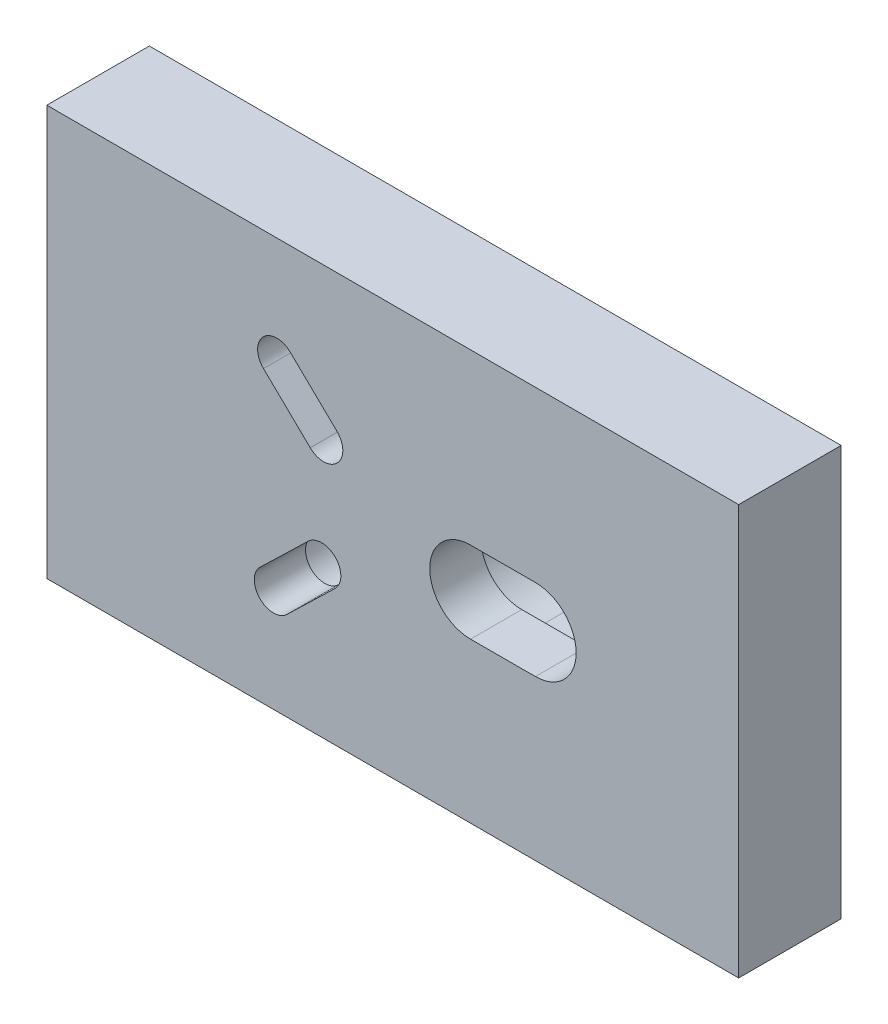
from build123d import *

# Parameters (mm, degrees)
SKETCH_1_W          = 27
SKETCH_1_H          = 16
EXTRUDE_1_DEPTH     = 4
SKETCH_2_R          = 0.75
SKETCH_2_R_2        = 1.59
CUT_EXTRUDE_2_DEPTH = 4
CUT_EXTRUDE_3_DEPTH = 4
CUT_EXTRUDE_4_DEPTH = 2


with BuildPart() as part:
    # 草图1 → 凸台-拉伸1 (new body)
    with BuildSketch(Plane.XY):
        with Locations((3.898916968, -3.881768953)):
            Rectangle(SKETCH_1_W, SKETCH_1_H)
    extrude(amount=EXTRUDE_1_DEPTH)

    # 草图2 → 切除-拉伸2 (cut)
    with BuildSketch(Plane.XY.offset(4)):
        with Locations((1.199905932, -1.781578746)):
            Circle(SKETCH_2_R)
        with Locations((1.122511443, -6.056778774)):
            Circle(SKETCH_2_R)
        with Locations((9.465404763, -4.069510677)):
            Circle(SKETCH_2_R_2)
    extrude(amount=-CUT_EXTRUDE_2_DEPTH, mode=Mode.SUBTRACT)

    # 草图3 → 切除-拉伸3 (cut)
    with BuildSketch(Plane.XY.offset(4)):
        with BuildLine():
            Line((6.931862452, -2.481455291), (9.464184068, -2.479511145))
            ThreePointArc((9.464184068, -2.479511145), (7.875405231, -4.070731371), (9.466625457, -5.659510208))
            Line((9.466625457, -5.659510208), (6.934303841, -5.661454354))
            ThreePointArc((6.934303841, -5.661454354), (5.343083615, -4.072675517), (6.931862452, -2.481455291))
        make_face()
        with BuildLine():
            Line((-1.276445305, -7.332757851), (0.601227077, -5.517554692))
            ThreePointArc((0.601227077, -5.517554692), (0.583287361, -6.578063139), (1.643795809, -6.596002856))
            Line((1.643795809, -6.596002856), (-0.233876574, -8.411206015))
            ThreePointArc((-0.233876574, -8.411206015), (-1.294385021, -8.393266299), (-1.276445305, -7.332757851))
        make_face()
        with BuildLine():
            Line((-1.145979965, -0.556904877), (0.678621567, -2.320802827))
            ThreePointArc((0.678621567, -2.320802827), (0.660681851, -1.26029438), (1.721190298, -1.242354664))
            Line((1.721190298, -1.242354664), (-0.103411234, 0.521543286))
            ThreePointArc((-0.103411234, 0.521543286), (-1.163919681, 0.50360357), (-1.145979965, -0.556904877))
        make_face()
    extrude(amount=-CUT_EXTRUDE_3_DEPTH, mode=Mode.SUBTRACT)

    # 草图5 → 切除-拉伸4 (cut)
    with BuildSketch(Plane(origin=(0, 0, 0), x_dir=(-1, 0, 0), z_dir=(0, 0, -1))):
        with BuildLine():
            Line((-9.463485432, -1.569511413), (-6.931163815, -1.57145556))
            ThreePointArc((-6.931163815, -1.57145556), (-4.433083883, -4.073374154), (-6.935002478, -6.571454086))
            Line((-6.935002478, -6.571454086), (-9.467324094, -6.56950994))
            ThreePointArc((-9.467324094, -6.56950994), (-11.965404026, -4.067591345), (-9.463485432, -1.569511413))
        make_face()
        with BuildLine():
            Line((-0.244111676, 0.881026007), (-2.068713208, -0.882871943))
            ThreePointArc((-2.068713208, -0.882871943), (-2.098612735, -2.650386022), (-0.331098657, -2.680285548))
            Line((-0.331098657, -2.680285548), (1.493502876, -0.916387599))
            ThreePointArc((1.493502876, -0.916387599), (1.523402402, 0.85112648), (-0.244111676, 0.881026007))
        make_face()
        with BuildLine():
            Line((-0.253704167, -5.158071971), (1.623968215, -6.97327513))
            ThreePointArc((1.623968215, -6.97327513), (1.653867742, -8.740789209), (-0.113646337, -8.770688736))
            Line((-0.113646337, -8.770688736), (-1.991318719, -6.955485577))
            ThreePointArc((-1.991318719, -6.955485577), (-2.021218246, -5.187971498), (-0.253704167, -5.158071971))
        make_face()
    extrude(amount=-CUT_EXTRUDE_4_DEPTH, mode=Mode.SUBTRACT)


solid = part.part
